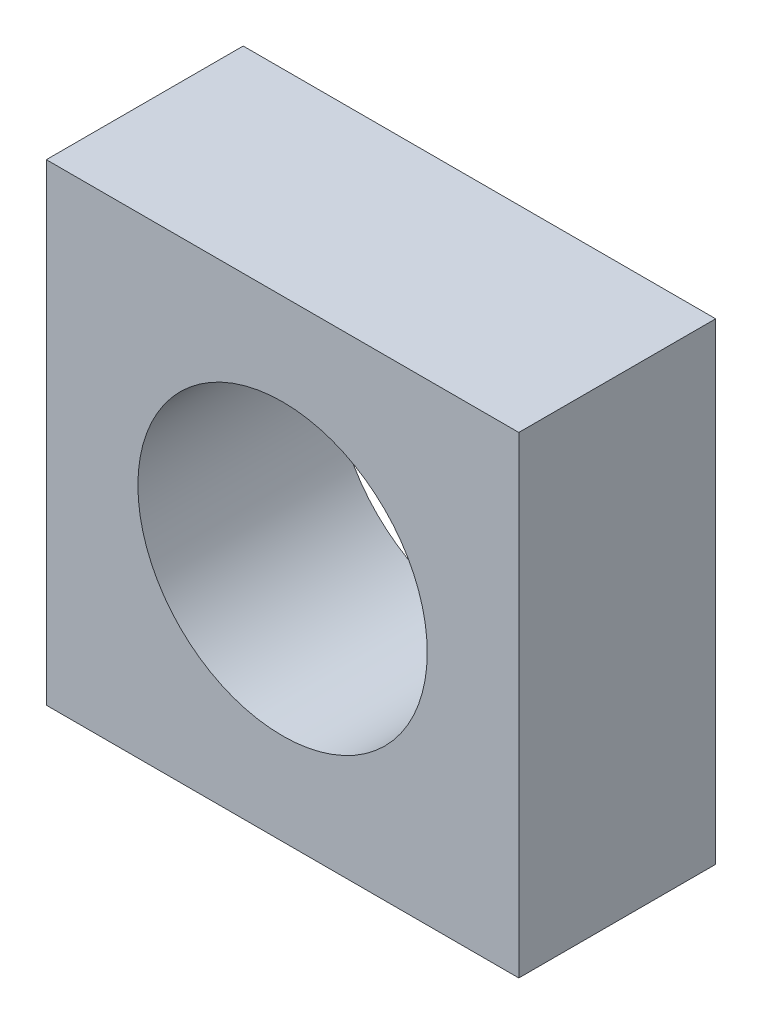
from build123d import *

# Parameters (mm, degrees)
SKETCH1_W           = 12
SKETCH1_H           = 12
SKETCH1_R           = 3.674588618
BOSS_EXTRUDE1_DEPTH = 5


with BuildPart() as part:
    # Sketch1 → Boss-Extrude1 (new body)
    with BuildSketch(Plane.XY):
        with Locations((-27.065651732, 0)):
            Rectangle(SKETCH1_W, SKETCH1_H)
        with Locations((-27.065651732, 0)):
            Circle(SKETCH1_R, mode=Mode.SUBTRACT)
    extrude(amount=-BOSS_EXTRUDE1_DEPTH)


solid = part.part
